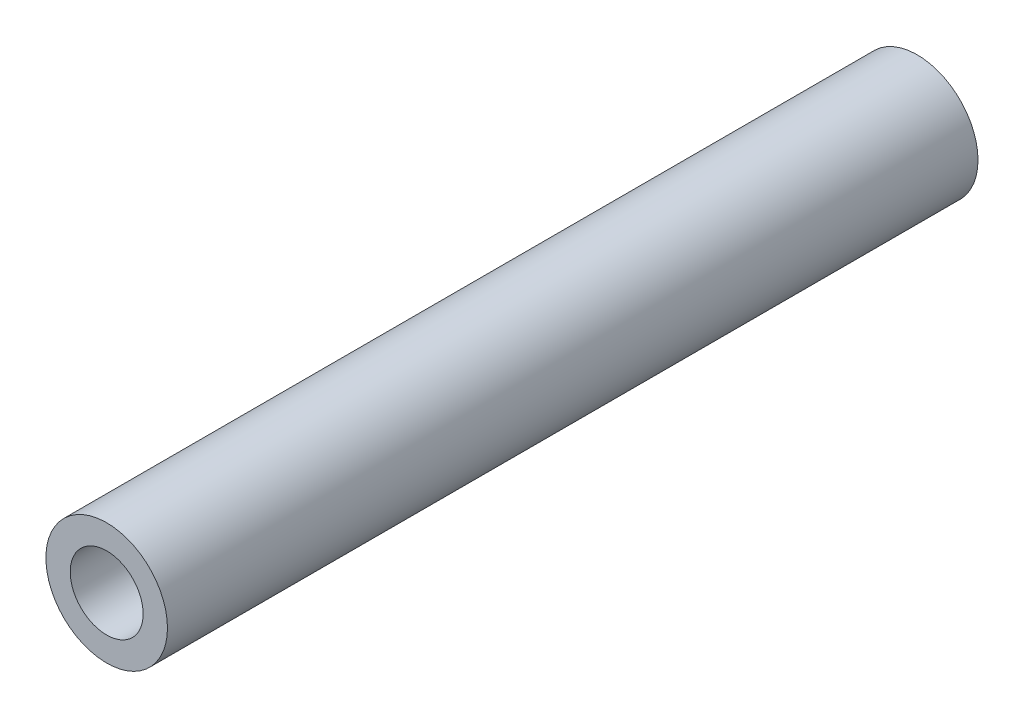
SolidWorks part; units mm, degrees
ref_plane "前视基准面" through (0, 0, 0) normal (0, 0, 1) x (1, 0, 0)
ref_plane "上视基准面" through (0, 0, 0) normal (0, 1, 0) x (1, 0, 0)
ref_plane "右视基准面" through (0, 0, 0) normal (1, 0, 0) x (0, 0, -1)
sketch "草图1" plane through (0, 0, 0) normal (0, 0, 1) x (1, 0, 0)
  circle A0 centre (0, 0) radius 1.5
  circle A1 centre (0, 0) radius 0.9
  dimension "D1" = 3
  dimension "D2" = 1.8
extrude "拉伸1" add sketch "草图1" along normal blind 20
